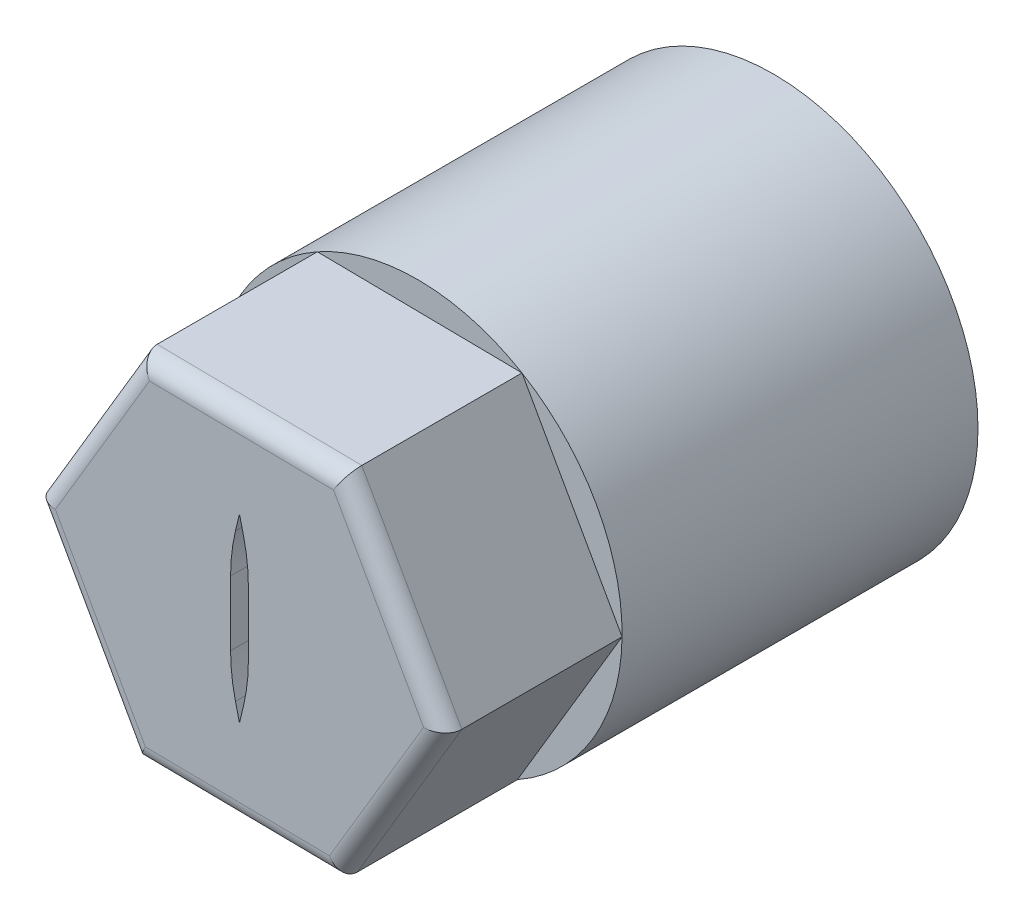
SolidWorks part; units mm, degrees
ref_plane "Front Plane" through (0, 0, 0) normal (0, 0, 1) x (1, 0, 0)
ref_plane "Top Plane" through (0, 0, 0) normal (0, 1, 0) x (1, 0, 0)
ref_plane "Right Plane" through (0, 0, 0) normal (1, 0, 0) x (0, 0, -1)
sketch "Sketch1" plane through (0, 0, 0) normal (0, 0, 1) x (1, 0, 0)
  circle A0 centre (0, 0) radius 11.5
extrude "Boss-Extrude1" add sketch "Sketch1" along normal blind 30
sketch "Sketch2" plane through (0, 0, 30) normal (0, 0, 1) x (1, 0, 0)
  line L1 (5.8758, 9.8856) -> (-5.6233, 10.0314)
  line L2 (-5.6233, 10.0314) -> (-11.4991, 0.1458)
  line L3 (-11.4991, 0.1458) -> (-5.8758, -9.8856)
  line L4 (-5.8758, -9.8856) -> (5.6233, -10.0314)
  line L5 (5.6233, -10.0314) -> (11.4991, -0.1458)
  line L6 (11.4991, -0.1458) -> (5.8758, 9.8856)
  circle A0 centre (0, 0) radius 9.9593 construction
extrude "Cut-Extrude2" cut sketch "Sketch2" against normal blind 10 flip side to cut
fillet "Fillet1" radius 1 6 edges at (-8.6874, -4.8699, 30) (-0.1262, -9.9585, 30) (8.5612, -5.0886, 30) (8.6874, 4.8699, 30) (0.1262, 9.9585, 30) (-8.5612, 5.0886, 30)
sketch "Sketch3" plane through (0, 0, 30) normal (0, 0, 1) x (1, 0, 0)
  line L4 (0.5, 0) -> (0.5, 1.8198)
  line L5 (0.5, 0) -> (0.5, -1.8198)
  line L6 (-0.5, 0) -> (-0.5, -1.8198)
  line L7 (-0.5, 0) -> (-0.5, 1.8198)
  line L8 (-0.2252, 4.1478) -> (0, 5.0887)
  line L9 (0, 5.0887) -> (0.2252, 4.1478)
  line L10 (0, -5.0887) -> (0.2252, -4.1478)
  line L11 (-0.2252, -4.1478) -> (0, -5.0887)
  arc A0 (0.2252, -4.1478) -> (0.5, -1.8198) centre (-9.5, -1.8198) ccw
  arc A1 (-0.5, -1.8198) -> (-0.2252, -4.1478) centre (9.5, -1.8198) ccw
  arc A2 (-0.5, 1.8198) -> (-0.2252, 4.1478) centre (9.5, 1.8198) cw
  arc A3 (0.5, 1.8198) -> (0.2252, 4.1478) centre (-9.5, 1.8198) ccw
  dimension "D1" = 10
extrude "Cut-Extrude3" cut sketch "Sketch3" against normal through all
sketch "Sketch4" plane through (0, 0, 0) normal (0, 0, -1) x (-1, 0, 0)
  circle A0 centre (0, 0) radius 10.5
extrude "Cut-Extrude4" cut sketch "Sketch4" against normal blind 18
